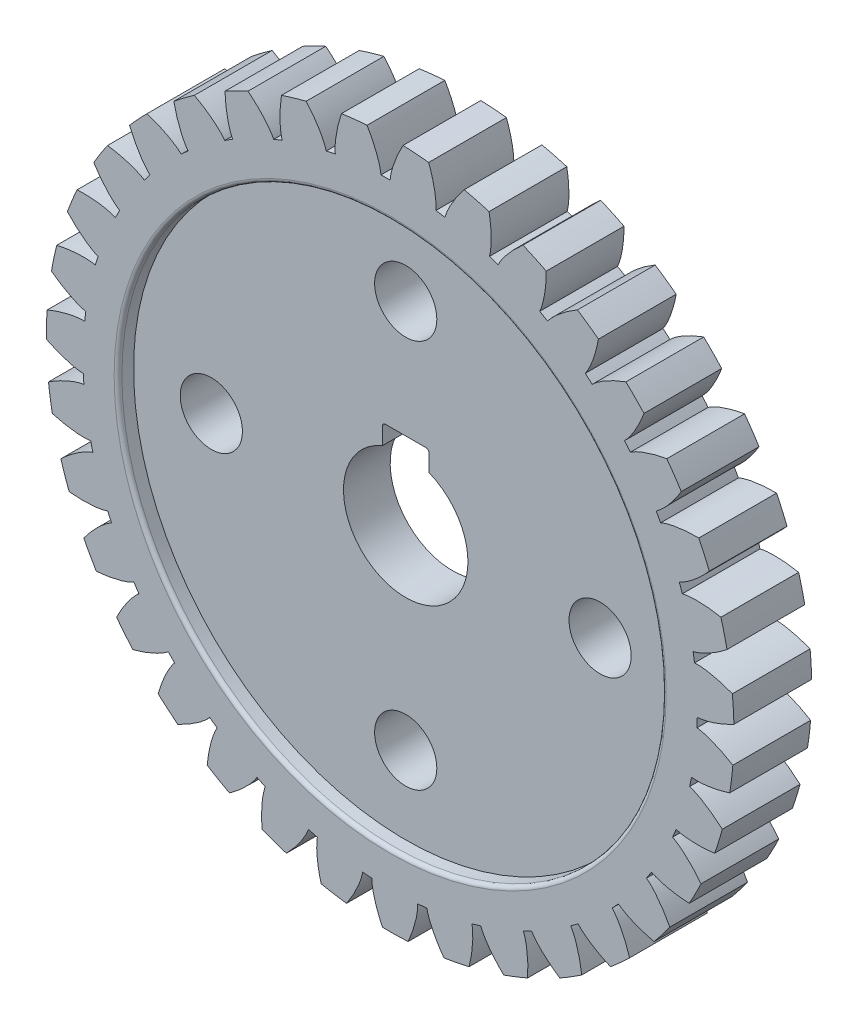
SolidWorks part; units mm, degrees
ref_plane "Front Plane" through (0, 0, 0) normal (0, 0, 1) x (1, 0, 0)
ref_plane "Top Plane" through (0, 0, 0) normal (0, 1, 0) x (1, 0, 0)
ref_plane "Right Plane" through (0, 0, 0) normal (1, 0, 0) x (0, 0, -1)
other "Configuration Table"
sketch "Sketch1" plane through (0, 0, 0) normal (0, 0, 1) x (1, 0, 0)
  line L0 (0, 22.1088) -> (0, 21) construction
  line L1 (0, 0) -> (0.8267, 22.0934) construction
  line L2 (0, 0) -> (2.4754, 21.9698) construction
  line L3 (0, 0) -> (1.6522, 22.047) construction
  line L4 (0, 0) -> (0, 14.7345) construction
  line L5 (0, 0) -> (4.1103, 21.7234) construction
  circle A0 centre (0, 0) radius 22.1088
  circle A1 centre (0, 0) radius 4
  circle A2 centre (0, 0) radius 19.75
  circle A3 centre (0, 0) radius 21 construction
  spline S0 degree 4 poles (0, 19.7335) (0.0004, 19.7495) (0.0024, 19.7944) (0.0107, 19.8789) (0.0304, 20.0163) (0.0799, 20.2697) (0.1609, 20.5699) (0.2731, 20.9038) (0.4141, 21.2564) (0.5474, 21.5537) (0.6917, 21.8458) (0.846, 22.1327) (1.0445, 22.4746) (1.2997, 22.8773) (1.62, 23.3348) (2.0126, 23.8396) (2.4375, 24.3344) (2.883, 24.8087) (3.3503, 25.2649) (3.8321, 25.6999) (4.3364, 26.1194) (4.7811, 26.4645) (5.1863, 26.7575) (5.5052, 26.9802) (5.8044, 27.1773) (6.0923, 27.3663) (6.5858, 27.6653) (6.8965, 27.8456) (7.3865, 28.1155) (7.5689, 28.2075) (7.7138, 28.2832) knots 0 0 0 0 0 0.005377 0.015084 0.028532 0.04661 0.092111 0.119476 0.146842 0.174209 0.201575 0.228941 0.256307 0.307035 0.361767 0.4165 0.471232 0.525964 0.580697 0.635429 0.690161 0.744894 0.77226 0.799626 0.826992 0.854358 0.909091 0.954545 1 1 1 1 1 construction
  spline S1 degree 4 poles (0.0005, 19.75) (0.001, 19.7619) (0.0033, 19.8026) (0.0113, 19.883) (0.0304, 20.0163) (0.0799, 20.2697) (0.1609, 20.5699) (0.2731, 20.9038) (0.4141, 21.2564) (0.5596, 21.5809) (0.6822, 21.8261) (0.7729, 21.9961) (0.8267, 22.0934) knots 0.001383 0.001383 0.001383 0.001383 0.001383 0.005377 0.015084 0.028532 0.04661 0.092111 0.119476 0.146842 0.174209 0.211577 0.211577 0.211577 0.211577 0.211577
  spline S2 degree 4 poles (2.9431, 19.5295) (2.9444, 19.5413) (2.9482, 19.5819) (2.9522, 19.6626) (2.9532, 19.7972) (2.942, 20.0552) (2.9067, 20.3641) (2.8455, 20.711) (2.7586, 21.0808) (2.6631, 21.4232) (2.5785, 21.684) (2.5141, 21.8656) (2.4754, 21.9698) knots 0.001383 0.001383 0.001383 0.001383 0.001383 0.005377 0.015084 0.028532 0.04661 0.092111 0.119476 0.146842 0.174209 0.211577 0.211577 0.211577 0.211577 0.211577
  spline S3 degree 4 poles (4.3953, 19.2547) (4.3984, 19.2662) (4.4097, 19.3054) (4.4354, 19.382) (4.4836, 19.5076) (4.5884, 19.7437) (4.7341, 20.0184) (4.9178, 20.3189) (5.1338, 20.6313) (5.3478, 20.9153) (5.5218, 21.1271) (5.6481, 21.2726) (5.7222, 21.3555) knots 0.001383 0.001383 0.001383 0.001383 0.001383 0.005377 0.015084 0.028532 0.04661 0.092111 0.119476 0.146842 0.174209 0.211577 0.211577 0.211577 0.211577 0.211577
  dimension "D1" = 2.143
  dimension "D2" = 8
  dimension "D3" = 4.286
  dimension "D4" = 42
  dimension "D5" = 6.429
  dimension "D7" = 39.5
  dimension "D6" = 6.429
sketch "Sketch4" plane through (0, 0, 0) normal (0, 0, 1) x (1, 0, 0)
  line L0 (0, 0) -> (4.1103, 21.7234) construction
  line L1 (0, 0) -> (0.7436, 3.9303) construction
  circle A0 centre (0, 0) radius 4 construction
  circle A1 centre (0, 0) radius 4
  arc A2 (0.0005, 19.75) -> (-0.5913, 19.7411) centre (0, 0) ccw
  circle A4 centre (0, 0) radius 19.75 construction
  arc A6 (2.4754, 21.9698) -> (0.8267, 22.0934) centre (0, 0) ccw
  arc A7 (-3.526, 19.4327) -> (-4.1068, 19.3183) centre (0, 0) ccw
  arc A8 (6.3585, 21.1747) -> (4.7583, 21.5907) centre (0, 0) ccw
  arc A9 (10.0372, 19.6991) -> (8.537, 20.3941) centre (0, 0) ccw
  arc A10 (13.3933, 17.5903) -> (12.0413, 18.542) centre (0, 0) ccw
  arc A11 (16.3189, 14.9162) -> (15.1586, 16.094) centre (0, 0) ccw
  arc A12 (18.7201, 11.7626) -> (17.7887, 13.1287) centre (0, 0) ccw
  arc A13 (20.5195, 8.231) -> (19.847, 9.7414) centre (0, 0) ccw
  arc A14 (21.6595, 4.4348) -> (21.2675, 6.041) centre (0, 0) ccw
  arc A15 (22.1032, 0.4961) -> (22.0044, 2.1465) centre (0, 0) ccw
  arc A16 (21.8366, -3.4586) -> (22.034, -1.8171) centre (0, 0) ccw
  arc A17 (20.8681, -7.3021) -> (21.3555, -5.7222) centre (0, 0) ccw
  arc A18 (19.2289, -10.9109) -> (19.9905, -9.4434) centre (0, 0) ccw
  arc A19 (16.9717, -14.169) -> (17.9831, -12.8611) centre (0, 0) ccw
  arc A20 (14.169, -16.9717) -> (15.3977, -15.8654) centre (0, 0) ccw
  arc A21 (10.9109, -19.2289) -> (12.3174, -18.3598) centre (0, 0) ccw
  arc A22 (7.3021, -20.8681) -> (8.8411, -20.2641) centre (0, 0) ccw
  arc A23 (3.4586, -21.8366) -> (5.0808, -21.5171) centre (0, 0) ccw
  arc A24 (-0.4961, -22.1032) -> (1.1571, -22.0785) centre (0, 0) ccw
  arc A25 (-4.4348, -21.6595) -> (-2.8038, -21.9303) centre (0, 0) ccw
  arc A26 (-8.231, -20.5195) -> (-6.6745, -21.0772) centre (0, 0) ccw
  arc A27 (-11.7626, -18.7201) -> (-10.3308, -19.5467) centre (0, 0) ccw
  arc A28 (-14.9162, -16.3189) -> (-13.6549, -17.388) centre (0, 0) ccw
  arc A29 (-17.5903, -13.3933) -> (-16.5402, -14.6704) centre (0, 0) ccw
  arc A30 (-19.6991, -10.0372) -> (-18.8939, -11.4812) centre (0, 0) ccw
  arc A31 (-21.1747, -6.3585) -> (-20.6404, -7.9231) centre (0, 0) ccw
  arc A32 (-21.9698, -2.4754) -> (-21.7234, -4.1103) centre (0, 0) ccw
  arc A33 (-22.0587, 1.4872) -> (-22.1082, -0.1654) centre (0, 0) ccw
  arc A34 (-21.4387, 5.4021) -> (-21.7824, 3.7849) centre (0, 0) ccw
  arc A35 (-20.1296, 9.1433) -> (-20.7566, 7.6134) centre (0, 0) ccw
  arc A36 (-18.1735, 12.5906) -> (-19.0636, 11.1973) centre (0, 0) ccw
  arc A37 (-15.6333, 15.6333) -> (-16.7579, 14.4213) centre (0, 0) ccw
  arc A38 (-12.5906, 18.1735) -> (-13.9135, 17.1818) centre (0, 0) ccw
  arc A39 (-9.1433, 20.1296) -> (-10.622, 19.39) centre (0, 0) ccw
  arc A40 (-5.4021, 21.4387) -> (-6.9891, 20.975) centre (0, 0) ccw
  arc A41 (-1.4872, 22.0587) -> (-3.1315, 21.8859) centre (0, 0) ccw
  arc A42 (3.527, 19.4325) -> (2.9431, 19.5295) centre (0, 0) ccw
  arc A43 (6.9401, 18.4905) -> (6.3829, 18.6901) centre (0, 0) ccw
  arc A44 (10.1302, 16.9541) -> (9.6176, 17.2501) centre (0, 0) ccw
  arc A45 (12.9947, 14.8728) -> (12.5431, 15.2556) centre (0, 0) ccw
  arc A46 (15.4415, 12.3135) -> (15.0656, 12.7707) centre (0, 0) ccw
  arc A47 (17.392, 9.3585) -> (17.1037, 9.8754) centre (0, 0) ccw
  arc A48 (18.7835, 6.1026) -> (18.5922, 6.6628) centre (0, 0) ccw
  arc A49 (19.5713, 2.6506) -> (19.4831, 3.2359) centre (0, 0) ccw
  arc A50 (19.7301, -0.8866) -> (19.7478, -0.2949) centre (0, 0) ccw
  arc A51 (19.2547, -4.3953) -> (19.3778, -3.8163) centre (0, 0) ccw
  arc A52 (18.1605, -7.7627) -> (18.3849, -7.215) centre (0, 0) ccw
  arc A53 (16.4825, -10.8806) -> (16.8012, -10.3818) centre (0, 0) ccw
  arc A54 (14.2748, -13.6489) -> (14.6775, -13.2149) centre (0, 0) ccw
  arc A55 (11.6083, -15.9784) -> (12.082, -15.6233) centre (0, 0) ccw
  arc A56 (8.5687, -17.7944) -> (9.0981, -17.5296) centre (0, 0) ccw
  arc A57 (5.2537, -19.0384) -> (5.8219, -18.8724) centre (0, 0) ccw
  arc A58 (1.7699, -19.6705) -> (2.3585, -19.6087) centre (0, 0) ccw
  arc A59 (-1.7709, -19.6704) -> (-1.1806, -19.7147) centre (0, 0) ccw
  arc A60 (-5.2547, -19.0381) -> (-4.6818, -19.187) centre (0, 0) ccw
  arc A61 (-8.5697, -17.7939) -> (-8.0326, -18.0427) centre (0, 0) ccw
  arc A62 (-11.6092, -15.9778) -> (-11.1251, -16.3185) centre (0, 0) ccw
  arc A63 (-14.2756, -13.6481) -> (-13.8601, -14.0698) centre (0, 0) ccw
  arc A64 (-16.4831, -10.8798) -> (-16.1497, -11.3689) centre (0, 0) ccw
  arc A65 (-18.1609, -7.7618) -> (-17.9201, -8.3025) centre (0, 0) ccw
  arc A66 (-19.2549, -4.3943) -> (-19.1146, -4.9693) centre (0, 0) ccw
  arc A67 (-19.7301, -0.8856) -> (-19.6947, -1.4764) centre (0, 0) ccw
  arc A68 (-19.5712, 2.6516) -> (-19.6419, 2.0639) centre (0, 0) ccw
  arc A69 (-18.7832, 6.1036) -> (-18.9577, 5.5379) centre (0, 0) ccw
  arc A70 (-17.3915, 9.3594) -> (-17.6642, 8.834) centre (0, 0) ccw
  arc A71 (-12.9939, 14.8735) -> (-13.4338, 14.4774) centre (0, 0) ccw
  arc A72 (-15.4409, 12.3143) -> (-15.8029, 11.8461) centre (0, 0) ccw
  arc A73 (-10.1293, 16.9546) -> (-10.6329, 16.6435) centre (0, 0) ccw
  arc A74 (-6.9392, 18.4908) -> (-7.4902, 18.2746) centre (0, 0) ccw
  spline S0 degree 4 poles (3.527, 19.4325) (3.5296, 19.4441) (3.5391, 19.4838) (3.5614, 19.5615) (3.6039, 19.6892) (3.6979, 19.9296) (3.8312, 20.2106) (4.0012, 20.5191) (4.203, 20.8409) (4.404, 21.1342) (4.5684, 21.3536) (4.688, 21.5046) (4.7583, 21.5907) knots 0.001383 0.001383 0.001383 0.001383 0.001383 0.005377 0.015084 0.028532 0.04661 0.092111 0.119476 0.146842 0.174209 0.211577 0.211577 0.211577 0.211577 0.211577
  spline S1 degree 4 poles (-1975.8072, 309.5897) (-30.9922, 20.4545) (1.9661, 17.0455) (2.9426, 18.3846) (2.9532, 19.7972) (2.942, 20.0552) (2.9067, 20.3641) (2.8455, 20.711) (2.7586, 21.0808) (0.373, 29.6398) (-13.398, 34.7339) (17.5347, 27.1799) (-1817.0292, 852.0524) knots -0.428025 -0.428025 -0.428025 -0.428025 -0.428025 0.005377 0.015084 0.028532 0.04661 0.092111 0.119476 0.146842 0.174209 3.077604 3.077604 3.077604 3.077604 3.077604 only from (2.9431, 19.5295) to (2.4754, 21.9698) construction
  spline S2 degree 4 poles (1999.881, 11.6531) (33.6946, 15.6069) (0.5963, 17.1482) (-0.1697, 18.6179) (0.0304, 20.0163) (0.0799, 20.2697) (0.1609, 20.5699) (0.2731, 20.9038) (0.4141, 21.2564) (4.0487, 29.3643) (18.4252, 32.3491) (-13.2879, 29.4898) (1923.7263, 571.7216) knots -0.428025 -0.428025 -0.428025 -0.428025 -0.428025 0.005377 0.015084 0.028532 0.04661 0.092111 0.119476 0.146842 0.174209 3.077604 3.077604 3.077604 3.077604 3.077604 only from (0.0005, 19.75) to (0.8267, 22.0934) construction
  spline S3 degree 4 poles (6.3829, 18.6901) (6.3863, 18.7015) (6.3973, 18.7408) (6.4157, 18.8195) (6.4407, 18.9517) (6.4757, 19.2076) (6.4962, 19.5178) (6.4979, 19.8701) (6.4784, 20.2494) (6.4456, 20.6034) (6.4089, 20.8751) (6.378, 21.0653) (6.3585, 21.1747) knots 0.001383 0.001383 0.001383 0.001383 0.001383 0.005377 0.015084 0.028532 0.04661 0.092111 0.119476 0.146842 0.174209 0.211577 0.211577 0.211577 0.211577 0.211577
  spline S4 degree 4 poles (2.9431, 19.5295) (2.9444, 19.5413) (2.9482, 19.5819) (2.9522, 19.6626) (2.9532, 19.7972) (2.942, 20.0552) (2.9067, 20.3641) (2.8455, 20.711) (2.7586, 21.0808) (2.6631, 21.4232) (2.5785, 21.684) (2.5141, 21.8656) (2.4754, 21.9698) knots 0.001383 0.001383 0.001383 0.001383 0.001383 0.005377 0.015084 0.028532 0.04661 0.092111 0.119476 0.146842 0.174209 0.211577 0.211577 0.211577 0.211577 0.211577
  spline S5 degree 4 poles (0.0005, 19.75) (0.001, 19.7619) (0.0033, 19.8026) (0.0113, 19.883) (0.0304, 20.0163) (0.0799, 20.2697) (0.1609, 20.5699) (0.2731, 20.9038) (0.4141, 21.2564) (0.5596, 21.5809) (0.6822, 21.8261) (0.7729, 21.9961) (0.8267, 22.0934) knots 0.001383 0.001383 0.001383 0.001383 0.001383 0.005377 0.015084 0.028532 0.04661 0.092111 0.119476 0.146842 0.174209 0.211577 0.211577 0.211577 0.211577 0.211577
  spline S6 degree 4 poles (6.9401, 18.4905) (6.9447, 18.5014) (6.9612, 18.5387) (6.997, 18.6112) (7.0616, 18.7292) (7.1971, 18.9491) (7.3783, 19.2017) (7.6007, 19.4749) (7.8567, 19.7555) (8.1069, 20.0082) (8.3078, 20.1947) (8.4524, 20.3219) (8.537, 20.3941) knots 0.001383 0.001383 0.001383 0.001383 0.001383 0.005377 0.015084 0.028532 0.04661 0.092111 0.119476 0.146842 0.174209 0.211577 0.211577 0.211577 0.211577 0.211577
  spline S7 degree 4 poles (9.6176, 17.2501) (9.6229, 17.2607) (9.6408, 17.2973) (9.6729, 17.3715) (9.7212, 17.4971) (9.8013, 17.7426) (9.8768, 18.0442) (9.9414, 18.3905) (9.9899, 18.7672) (10.0209, 19.1214) (10.0333, 19.3953) (10.0368, 19.5879) (10.0372, 19.6991) knots 0.001383 0.001383 0.001383 0.001383 0.001383 0.005377 0.015084 0.028532 0.04661 0.092111 0.119476 0.146842 0.174209 0.211577 0.211577 0.211577 0.211577 0.211577
  spline S8 degree 4 poles (10.1302, 16.9541) (10.1367, 16.9641) (10.1595, 16.9978) (10.2077, 17.0627) (10.2924, 17.1673) (10.4649, 17.3595) (10.6884, 17.5757) (10.956, 17.8048) (11.2579, 18.0352) (11.5492, 18.2391) (11.7802, 18.3867) (11.9452, 18.4861) (12.0413, 18.542) knots 0.001383 0.001383 0.001383 0.001383 0.001383 0.005377 0.015084 0.028532 0.04661 0.092111 0.119476 0.146842 0.174209 0.211577 0.211577 0.211577 0.211577 0.211577
  spline S9 degree 4 poles (12.5431, 15.2556) (12.5503, 15.265) (12.5744, 15.2979) (12.6193, 15.3652) (12.6892, 15.4802) (12.8118, 15.7074) (12.94, 15.9907) (13.0654, 16.3199) (13.1804, 16.6819) (13.2741, 17.0248) (13.3352, 17.2921) (13.3731, 17.481) (13.3933, 17.5903) knots 0.001383 0.001383 0.001383 0.001383 0.001383 0.005377 0.015084 0.028532 0.04661 0.092111 0.119476 0.146842 0.174209 0.211577 0.211577 0.211577 0.211577 0.211577
  spline S10 degree 4 poles (12.9947, 14.8728) (13.0028, 14.8815) (13.0313, 14.9106) (13.0903, 14.9659) (13.1923, 15.0537) (13.3964, 15.2119) (13.6549, 15.3848) (13.9591, 15.5624) (14.2973, 15.7351) (14.6203, 15.8838) (14.874, 15.9878) (15.0541, 16.0561) (15.1586, 16.094) knots 0.001383 0.001383 0.001383 0.001383 0.001383 0.005377 0.015084 0.028532 0.04661 0.092111 0.119476 0.146842 0.174209 0.211577 0.211577 0.211577 0.211577 0.211577
  spline S11 degree 4 poles (15.0656, 12.7707) (15.0743, 12.7788) (15.1039, 12.8068) (15.16, 12.865) (15.2493, 12.9657) (15.4106, 13.1673) (15.5873, 13.4232) (15.7695, 13.7247) (15.9473, 14.0603) (16.1007, 14.3811) (16.2085, 14.6331) (16.2795, 14.8122) (16.3189, 14.9162) knots 0.001383 0.001383 0.001383 0.001383 0.001383 0.005377 0.015084 0.028532 0.04661 0.092111 0.119476 0.146842 0.174209 0.211577 0.211577 0.211577 0.211577 0.211577
  spline S12 degree 4 poles (15.4415, 12.3135) (15.4511, 12.3206) (15.4843, 12.3442) (15.5522, 12.388) (15.6683, 12.4562) (15.8973, 12.5754) (16.1825, 12.6994) (16.5135, 12.8198) (16.8772, 12.9294) (17.2215, 13.018) (17.4897, 13.075) (17.6791, 13.1101) (17.7887, 13.1287) knots 0.001383 0.001383 0.001383 0.001383 0.001383 0.005377 0.015084 0.028532 0.04661 0.092111 0.119476 0.146842 0.174209 0.211577 0.211577 0.211577 0.211577 0.211577
  spline S13 degree 4 poles (17.1037, 9.8754) (17.1138, 9.8818) (17.1479, 9.9041) (17.2135, 9.9513) (17.3194, 10.0344) (17.5141, 10.2041) (17.7336, 10.4242) (17.9667, 10.6884) (18.2015, 10.9869) (18.4098, 11.2751) (18.5609, 11.5038) (18.6627, 11.6673) (18.7201, 11.7626) knots 0.001383 0.001383 0.001383 0.001383 0.001383 0.005377 0.015084 0.028532 0.04661 0.092111 0.119476 0.146842 0.174209 0.211577 0.211577 0.211577 0.211577 0.211577
  spline S14 degree 4 poles (17.392, 9.3585) (17.4027, 9.3637) (17.4396, 9.3809) (17.5142, 9.412) (17.6406, 9.4583) (17.8873, 9.5348) (18.19, 9.6058) (18.5372, 9.6652) (18.9146, 9.7081) (19.2692, 9.7337) (19.5432, 9.742) (19.7359, 9.7427) (19.847, 9.7414) knots 0.001383 0.001383 0.001383 0.001383 0.001383 0.005377 0.015084 0.028532 0.04661 0.092111 0.119476 0.146842 0.174209 0.211577 0.211577 0.211577 0.211577 0.211577
  spline S15 degree 4 poles (18.5922, 6.6628) (18.6032, 6.6672) (18.6408, 6.6831) (18.7138, 6.7178) (18.8328, 6.7807) (19.0546, 6.9128) (19.31, 7.0903) (19.5864, 7.3086) (19.8708, 7.5603) (20.1272, 7.8067) (20.3167, 8.0048) (20.4461, 8.1475) (20.5195, 8.231) knots 0.001383 0.001383 0.001383 0.001383 0.001383 0.005377 0.015084 0.028532 0.04661 0.092111 0.119476 0.146842 0.174209 0.211577 0.211577 0.211577 0.211577 0.211577
  spline S16 degree 4 poles (18.7835, 6.1026) (18.795, 6.1058) (18.8344, 6.1162) (18.9134, 6.1334) (19.046, 6.1565) (19.3023, 6.1877) (19.6128, 6.2035) (19.9651, 6.1999) (20.3441, 6.1747) (20.6976, 6.1367) (20.9687, 6.0959) (21.1583, 6.0621) (21.2675, 6.041) knots 0.001383 0.001383 0.001383 0.001383 0.001383 0.005377 0.015084 0.028532 0.04661 0.092111 0.119476 0.146842 0.174209 0.211577 0.211577 0.211577 0.211577 0.211577
  spline S17 degree 4 poles (19.4831, 3.2359) (19.4947, 3.2383) (19.5345, 3.2472) (19.6125, 3.2684) (19.7409, 3.309) (19.9827, 3.3994) (20.2657, 3.5284) (20.5767, 3.6938) (20.9014, 3.8907) (21.1977, 4.0874) (21.4195, 4.2485) (21.5723, 4.3658) (21.6595, 4.4348) knots 0.001383 0.001383 0.001383 0.001383 0.001383 0.005377 0.015084 0.028532 0.04661 0.092111 0.119476 0.146842 0.174209 0.211577 0.211577 0.211577 0.211577 0.211577
  spline S18 degree 4 poles (19.5713, 2.6506) (19.5832, 2.6517) (19.6238, 2.6549) (19.7046, 2.6578) (19.8392, 2.6567) (20.0969, 2.6417) (20.4053, 2.6018) (20.7513, 2.5354) (21.1197, 2.4429) (21.4607, 2.3423) (21.7202, 2.2538) (21.9007, 2.1867) (22.0044, 2.1465) knots 0.001383 0.001383 0.001383 0.001383 0.001383 0.005377 0.015084 0.028532 0.04661 0.092111 0.119476 0.146842 0.174209 0.211577 0.211577 0.211577 0.211577 0.211577
  spline S19 degree 4 poles (19.7478, -0.2949) (19.7597, -0.2946) (19.8004, -0.293) (19.8809, -0.2861) (20.0145, -0.2691) (20.2686, -0.2233) (20.57, -0.1469) (20.9055, -0.0396) (21.2603, 0.0961) (21.5868, 0.2367) (21.8339, 0.3556) (22.0052, 0.4437) (22.1032, 0.4961) knots 0.001383 0.001383 0.001383 0.001383 0.001383 0.005377 0.015084 0.028532 0.04661 0.092111 0.119476 0.146842 0.174209 0.211577 0.211577 0.211577 0.211577 0.211577
  spline S20 degree 4 poles (19.7301, -0.8866) (19.7419, -0.8876) (19.7825, -0.8917) (19.8625, -0.9033) (19.9947, -0.9284) (20.2457, -0.9892) (20.542, -1.0836) (20.8705, -1.2107) (21.2165, -1.3674) (21.534, -1.5272) (21.7735, -1.6607) (21.9392, -1.7589) (22.034, -1.8171) knots 0.001383 0.001383 0.001383 0.001383 0.001383 0.005377 0.015084 0.028532 0.04661 0.092111 0.119476 0.146842 0.174209 0.211577 0.211577 0.211577 0.211577 0.211577
  spline S21 degree 4 poles (19.3778, -3.8163) (19.3895, -3.8181) (19.4299, -3.8238) (19.5104, -3.8314) (19.6448, -3.8385) (19.903, -3.8388) (20.2132, -3.8174) (20.5625, -3.7718) (20.9358, -3.7016) (21.2822, -3.6216) (21.5465, -3.5487) (21.7307, -3.4926) (21.8366, -3.4586) knots 0.001383 0.001383 0.001383 0.001383 0.001383 0.005377 0.015084 0.028532 0.04661 0.092111 0.119476 0.146842 0.174209 0.211577 0.211577 0.211577 0.211577 0.211577
  spline S22 degree 4 poles (19.2547, -4.3953) (19.2662, -4.3984) (19.3054, -4.4097) (19.382, -4.4354) (19.5076, -4.4836) (19.7437, -4.5884) (20.0184, -4.7341) (20.3189, -4.9178) (20.6313, -5.1338) (20.9153, -5.3478) (21.1271, -5.5218) (21.2726, -5.6481) (21.3555, -5.7222) knots 0.001383 0.001383 0.001383 0.001383 0.001383 0.005377 0.015084 0.028532 0.04661 0.092111 0.119476 0.146842 0.174209 0.211577 0.211577 0.211577 0.211577 0.211577
  spline S23 degree 4 poles (18.3849, -7.215) (18.3962, -7.2189) (18.4349, -7.2317) (18.5127, -7.2535) (18.6437, -7.2845) (18.8977, -7.3309) (19.2067, -7.3653) (19.5586, -7.3828) (19.9384, -7.3803) (20.2935, -7.3635) (20.5666, -7.339) (20.7579, -7.3166) (20.8681, -7.3021) knots 0.001383 0.001383 0.001383 0.001383 0.001383 0.005377 0.015084 0.028532 0.04661 0.092111 0.119476 0.146842 0.174209 0.211577 0.211577 0.211577 0.211577 0.211577
  spline S24 degree 4 poles (18.1605, -7.7627) (18.1712, -7.7678) (18.2077, -7.7859) (18.2785, -7.8249) (18.3936, -7.8948) (18.6071, -8.04) (18.8514, -8.2324) (19.1143, -8.4668) (19.3831, -8.7351) (19.6243, -8.9964) (19.8016, -9.2055) (19.9222, -9.3557) (19.9905, -9.4434) knots 0.001383 0.001383 0.001383 0.001383 0.001383 0.005377 0.015084 0.028532 0.04661 0.092111 0.119476 0.146842 0.174209 0.211577 0.211577 0.211577 0.211577 0.211577
  spline S25 degree 4 poles (16.8012, -10.3818) (16.8116, -10.3877) (16.8474, -10.4071) (16.92, -10.4425) (17.0434, -10.4964) (17.285, -10.5874) (17.583, -10.6764) (17.926, -10.7565) (18.3001, -10.8219) (18.6526, -10.8687) (18.9256, -10.8933) (19.1179, -10.9055) (19.2289, -10.9109) knots 0.001383 0.001383 0.001383 0.001383 0.001383 0.005377 0.015084 0.028532 0.04661 0.092111 0.119476 0.146842 0.174209 0.211577 0.211577 0.211577 0.211577 0.211577
  spline S26 degree 4 poles (16.4825, -10.8806) (16.4922, -10.8876) (16.5249, -10.9119) (16.5876, -10.9629) (16.6883, -11.0522) (16.8725, -11.2332) (17.0785, -11.4661) (17.2953, -11.7438) (17.5119, -12.0557) (17.7026, -12.3559) (17.8397, -12.5933) (17.9315, -12.7626) (17.9831, -12.8611) knots 0.001383 0.001383 0.001383 0.001383 0.001383 0.005377 0.015084 0.028532 0.04661 0.092111 0.119476 0.146842 0.174209 0.211577 0.211577 0.211577 0.211577 0.211577
  spline S27 degree 4 poles (14.6775, -13.2149) (14.6866, -13.2225) (14.7184, -13.2481) (14.7835, -13.2959) (14.8953, -13.3709) (15.1168, -13.5037) (15.394, -13.6444) (15.7173, -13.7844) (16.0737, -13.9156) (16.4122, -14.0246) (16.6764, -14.0976) (16.8634, -14.1439) (16.9717, -14.169) knots 0.001383 0.001383 0.001383 0.001383 0.001383 0.005377 0.015084 0.028532 0.04661 0.092111 0.119476 0.146842 0.174209 0.211577 0.211577 0.211577 0.211577 0.211577
  spline S28 degree 4 poles (14.2748, -13.6489) (14.2831, -13.6574) (14.3109, -13.6872) (14.3635, -13.7486) (14.4467, -13.8544) (14.5956, -14.0654) (14.7567, -14.3313) (14.9204, -14.6432) (15.0778, -14.9889) (15.2118, -15.3182) (15.3044, -15.5763) (15.3645, -15.7593) (15.3977, -15.8654) knots 0.001383 0.001383 0.001383 0.001383 0.001383 0.005377 0.015084 0.028532 0.04661 0.092111 0.119476 0.146842 0.174209 0.211577 0.211577 0.211577 0.211577 0.211577
  spline S29 degree 4 poles (12.082, -15.6233) (12.0896, -15.6324) (12.1163, -15.6632) (12.1719, -15.7219) (12.2685, -15.8157) (12.4627, -15.9858) (12.7104, -16.1738) (13.0034, -16.3693) (13.3307, -16.562) (13.6442, -16.7297) (13.8912, -16.8487) (14.0669, -16.9277) (14.169, -16.9717) knots 0.001383 0.001383 0.001383 0.001383 0.001383 0.005377 0.015084 0.028532 0.04661 0.092111 0.119476 0.146842 0.174209 0.211577 0.211577 0.211577 0.211577 0.211577
  spline S30 degree 4 poles (11.6083, -15.9784) (11.6149, -15.9883) (11.637, -16.0225) (11.6778, -16.0923) (11.7407, -16.2113) (11.8495, -16.4455) (11.9605, -16.7359) (12.066, -17.072) (12.1592, -17.4403) (12.2322, -17.7882) (12.2772, -18.0587) (12.3037, -18.2495) (12.3174, -18.3598) knots 0.001383 0.001383 0.001383 0.001383 0.001383 0.005377 0.015084 0.028532 0.04661 0.092111 0.119476 0.146842 0.174209 0.211577 0.211577 0.211577 0.211577 0.211577
  spline S31 degree 4 poles (9.0981, -17.5296) (9.104, -17.5399) (9.1248, -17.575) (9.169, -17.6427) (9.2473, -17.7521) (9.408, -17.9542) (9.6181, -18.1834) (9.8716, -18.4281) (10.1592, -18.6761) (10.4378, -18.8971) (10.6595, -19.0583) (10.8183, -19.1674) (10.9109, -19.2289) knots 0.001383 0.001383 0.001383 0.001383 0.001383 0.005377 0.015084 0.028532 0.04661 0.092111 0.119476 0.146842 0.174209 0.211577 0.211577 0.211577 0.211577 0.211577
  spline S32 degree 4 poles (8.5687, -17.7944) (8.5735, -17.8053) (8.5891, -17.8429) (8.6167, -17.9189) (8.6574, -18.0472) (8.7227, -18.297) (8.78, -18.6026) (8.8238, -18.9522) (8.8497, -19.3311) (8.8594, -19.6865) (8.8554, -19.9606) (8.8474, -20.1531) (8.8411, -20.2641) knots 0.001383 0.001383 0.001383 0.001383 0.001383 0.005377 0.015084 0.028532 0.04661 0.092111 0.119476 0.146842 0.174209 0.211577 0.211577 0.211577 0.211577 0.211577
  spline S33 degree 4 poles (5.8219, -18.8724) (5.8259, -18.8836) (5.84, -18.9218) (5.8714, -18.9963) (5.9289, -19.118) (6.051, -19.3456) (6.2168, -19.6086) (6.4225, -19.8946) (6.6612, -20.19) (6.8958, -20.4572) (7.0852, -20.6554) (7.222, -20.791) (7.3021, -20.8681) knots 0.001383 0.001383 0.001383 0.001383 0.001383 0.005377 0.015084 0.028532 0.04661 0.092111 0.119476 0.146842 0.174209 0.211577 0.211577 0.211577 0.211577 0.211577
  spline S34 degree 4 poles (5.2537, -19.0384) (5.2564, -19.05) (5.2651, -19.0898) (5.2787, -19.1695) (5.2958, -19.303) (5.3154, -19.5605) (5.3173, -19.8714) (5.2979, -20.2231) (5.2558, -20.6006) (5.2019, -20.952) (5.149, -21.221) (5.1068, -21.409) (5.0808, -21.5171) knots 0.001383 0.001383 0.001383 0.001383 0.001383 0.005377 0.015084 0.028532 0.04661 0.092111 0.119476 0.146842 0.174209 0.211577 0.211577 0.211577 0.211577 0.211577
  spline S35 degree 4 poles (2.3585, -19.6087) (2.3604, -19.6204) (2.3675, -19.6605) (2.3851, -19.7394) (2.42, -19.8694) (2.4994, -20.1151) (2.6156, -20.4035) (2.7669, -20.7217) (2.9491, -21.0549) (3.1322, -21.3597) (3.2832, -21.5885) (3.3935, -21.7464) (3.4586, -21.8366) knots 0.001383 0.001383 0.001383 0.001383 0.001383 0.005377 0.015084 0.028532 0.04661 0.092111 0.119476 0.146842 0.174209 0.211577 0.211577 0.211577 0.211577 0.211577
  spline S36 degree 4 poles (1.7699, -19.6705) (1.7705, -19.6824) (1.7718, -19.7231) (1.771, -19.804) (1.764, -19.9384) (1.7373, -20.1952) (1.6837, -20.5015) (1.6018, -20.8441) (1.4929, -21.208) (1.3772, -21.5442) (1.2771, -21.7994) (1.202, -21.9768) (1.1571, -22.0785) knots 0.001383 0.001383 0.001383 0.001383 0.001383 0.005377 0.015084 0.028532 0.04661 0.092111 0.119476 0.146842 0.174209 0.211577 0.211577 0.211577 0.211577 0.211577
  spline S37 degree 4 poles (-1.1806, -19.7147) (-1.1809, -19.7266) (-1.181, -19.7673) (-1.1778, -19.8481) (-1.1667, -19.9822) (-1.1324, -20.2382) (-1.0696, -20.5427) (-0.9775, -20.8827) (-0.8578, -21.2432) (-0.732, -21.5757) (-0.6244, -21.8278) (-0.544, -22.0029) (-0.4961, -22.1032) knots 0.001383 0.001383 0.001383 0.001383 0.001383 0.005377 0.015084 0.028532 0.04661 0.092111 0.119476 0.146842 0.174209 0.211577 0.211577 0.211577 0.211577 0.211577
  spline S38 degree 4 poles (-1.7709, -19.6704) (-1.7724, -19.6822) (-1.7783, -19.7226) (-1.7936, -19.8019) (-1.8245, -19.9329) (-1.8966, -20.1809) (-2.0041, -20.4727) (-2.1458, -20.7952) (-2.3179, -21.1337) (-2.4918, -21.4438) (-2.6359, -21.6771) (-2.7415, -21.8382) (-2.8038, -21.9303) knots 0.001383 0.001383 0.001383 0.001383 0.001383 0.005377 0.015084 0.028532 0.04661 0.092111 0.119476 0.146842 0.174209 0.211577 0.211577 0.211577 0.211577 0.211577
  spline S39 degree 4 poles (-4.6818, -19.187) (-4.6842, -19.1987) (-4.6916, -19.2388) (-4.7029, -19.3188) (-4.716, -19.4528) (-4.7279, -19.7107) (-4.7205, -20.0216) (-4.6906, -20.3726) (-4.6371, -20.7486) (-4.5728, -21.0983) (-4.5118, -21.3656) (-4.464, -21.5522) (-4.4348, -21.6595) knots 0.001383 0.001383 0.001383 0.001383 0.001383 0.005377 0.015084 0.028532 0.04661 0.092111 0.119476 0.146842 0.174209 0.211577 0.211577 0.211577 0.211577 0.211577
  spline S40 degree 4 poles (-5.2547, -19.0381) (-5.2583, -19.0494) (-5.2714, -19.0881) (-5.3005, -19.1635) (-5.3543, -19.2868) (-5.4695, -19.5179) (-5.6274, -19.7858) (-5.8244, -20.0778) (-6.0542, -20.3802) (-6.2807, -20.6543) (-6.4641, -20.8581) (-6.5968, -20.9978) (-6.6745, -21.0772) knots 0.001383 0.001383 0.001383 0.001383 0.001383 0.005377 0.015084 0.028532 0.04661 0.092111 0.119476 0.146842 0.174209 0.211577 0.211577 0.211577 0.211577 0.211577
  spline S41 degree 4 poles (-8.0326, -18.0427) (-8.037, -18.0538) (-8.0515, -18.0919) (-8.0768, -18.1686) (-8.1136, -18.2981) (-8.1714, -18.5498) (-8.2196, -18.857) (-8.2529, -19.2076) (-8.2674, -19.5872) (-8.2665, -19.9427) (-8.2543, -20.2166) (-8.2406, -20.4087) (-8.231, -20.5195) knots 0.001383 0.001383 0.001383 0.001383 0.001383 0.005377 0.015084 0.028532 0.04661 0.092111 0.119476 0.146842 0.174209 0.211577 0.211577 0.211577 0.211577 0.211577
  spline S42 degree 4 poles (-8.5697, -17.7939) (-8.5752, -17.8044) (-8.595, -17.8401) (-8.6371, -17.9091) (-8.7121, -18.0208) (-8.8667, -18.2277) (-9.0699, -18.463) (-9.3159, -18.7152) (-9.596, -18.9717) (-9.8678, -19.2009) (-10.0846, -19.3687) (-10.2401, -19.4824) (-10.3308, -19.5467) knots 0.001383 0.001383 0.001383 0.001383 0.001383 0.005377 0.015084 0.028532 0.04661 0.092111 0.119476 0.146842 0.174209 0.211577 0.211577 0.211577 0.211577 0.211577
  spline S43 degree 4 poles (-11.1251, -16.3185) (-11.1314, -16.3286) (-11.1525, -16.3635) (-11.1911, -16.4345) (-11.2505, -16.5553) (-11.3523, -16.7926) (-11.4545, -17.0863) (-11.5499, -17.4254) (-11.632, -17.7962) (-11.6946, -18.1462) (-11.7315, -18.4179) (-11.7522, -18.6094) (-11.7626, -18.7201) knots 0.001383 0.001383 0.001383 0.001383 0.001383 0.005377 0.015084 0.028532 0.04661 0.092111 0.119476 0.146842 0.174209 0.211577 0.211577 0.211577 0.211577 0.211577
  spline S44 degree 4 poles (-11.6092, -15.9778) (-11.6165, -15.9871) (-11.6423, -16.0187) (-11.6961, -16.079) (-11.7898, -16.1756) (-11.9789, -16.3515) (-12.2208, -16.5468) (-12.5079, -16.751) (-12.8293, -16.9534) (-13.1376, -17.1304) (-13.3809, -17.2567) (-13.5542, -17.3409) (-13.6549, -17.388) knots 0.001383 0.001383 0.001383 0.001383 0.001383 0.005377 0.015084 0.028532 0.04661 0.092111 0.119476 0.146842 0.174209 0.211577 0.211577 0.211577 0.211577 0.211577
  spline S45 degree 4 poles (-13.8601, -14.0698) (-13.8681, -14.0786) (-13.8951, -14.1092) (-13.9458, -14.1721) (-14.0257, -14.2804) (-14.1683, -14.4957) (-14.3213, -14.7664) (-14.4757, -15.083) (-14.6227, -15.4332) (-14.7468, -15.7664) (-14.8316, -16.0271) (-14.8862, -16.2119) (-14.9162, -16.3189) knots 0.001383 0.001383 0.001383 0.001383 0.001383 0.005377 0.015084 0.028532 0.04661 0.092111 0.119476 0.146842 0.174209 0.211577 0.211577 0.211577 0.211577 0.211577
  spline S46 degree 4 poles (-14.2756, -13.6481) (-14.2845, -13.656) (-14.3154, -13.6825) (-14.3791, -13.7322) (-14.4886, -13.8105) (-14.706, -13.9498) (-14.979, -14.0988) (-15.2979, -14.2484) (-15.6503, -14.3902) (-15.9853, -14.5093) (-16.2472, -14.5902) (-16.4327, -14.642) (-16.5402, -14.6704) knots 0.001383 0.001383 0.001383 0.001383 0.001383 0.005377 0.015084 0.028532 0.04661 0.092111 0.119476 0.146842 0.174209 0.211577 0.211577 0.211577 0.211577 0.211577
  spline S47 degree 4 poles (-16.1497, -11.3689) (-16.1591, -11.3761) (-16.1911, -11.4014) (-16.2522, -11.4542) (-16.3502, -11.5465) (-16.5289, -11.7329) (-16.7278, -11.9719) (-16.9362, -12.2559) (-17.1434, -12.5742) (-17.325, -12.8799) (-17.455, -13.1213) (-17.5417, -13.2933) (-17.5903, -13.3933) knots 0.001383 0.001383 0.001383 0.001383 0.001383 0.005377 0.015084 0.028532 0.04661 0.092111 0.119476 0.146842 0.174209 0.211577 0.211577 0.211577 0.211577 0.211577
  spline S48 degree 4 poles (-16.4831, -10.8798) (-16.4933, -10.8859) (-16.5285, -10.9065) (-16.6001, -10.944) (-16.7218, -11.0015) (-16.9606, -11.0998) (-17.2557, -11.1976) (-17.5962, -11.2879) (-17.9682, -11.3645) (-18.3191, -11.4218) (-18.5913, -11.4546) (-18.7831, -11.4725) (-18.8939, -11.4812) knots 0.001383 0.001383 0.001383 0.001383 0.001383 0.005377 0.015084 0.028532 0.04661 0.092111 0.119476 0.146842 0.174209 0.211577 0.211577 0.211577 0.211577 0.211577
  spline S49 degree 4 poles (-17.9201, -8.3025) (-17.9307, -8.3079) (-17.9667, -8.3271) (-18.0363, -8.3682) (-18.1492, -8.4415) (-18.3583, -8.593) (-18.5967, -8.7927) (-18.8525, -9.0349) (-19.1131, -9.3111) (-19.3464, -9.5794) (-19.5174, -9.7937) (-19.6334, -9.9475) (-19.6991, -10.0372) knots 0.001383 0.001383 0.001383 0.001383 0.001383 0.005377 0.015084 0.028532 0.04661 0.092111 0.119476 0.146842 0.174209 0.211577 0.211577 0.211577 0.211577 0.211577
  spline S50 degree 4 poles (-18.1609, -7.7618) (-18.172, -7.766) (-18.2103, -7.7799) (-18.2874, -7.8041) (-18.4174, -7.839) (-18.6699, -7.893) (-18.9778, -7.9366) (-19.329, -7.9646) (-19.7087, -7.9735) (-20.0642, -7.9673) (-20.3378, -7.9509) (-20.5297, -7.9343) (-20.6404, -7.9231) knots 0.001383 0.001383 0.001383 0.001383 0.001383 0.005377 0.015084 0.028532 0.04661 0.092111 0.119476 0.146842 0.174209 0.211577 0.211577 0.211577 0.211577 0.211577
  spline S51 degree 4 poles (-19.1146, -4.9693) (-19.126, -4.9728) (-19.1648, -4.9852) (-19.2406, -5.0132) (-19.3648, -5.0652) (-19.5976, -5.1769) (-19.8678, -5.3308) (-20.1627, -5.5234) (-20.4685, -5.7487) (-20.7459, -5.9711) (-20.9524, -6.1514) (-21.0941, -6.2819) (-21.1747, -6.3585) knots 0.001383 0.001383 0.001383 0.001383 0.001383 0.005377 0.015084 0.028532 0.04661 0.092111 0.119476 0.146842 0.174209 0.211577 0.211577 0.211577 0.211577 0.211577
  spline S52 degree 4 poles (-19.2549, -4.3943) (-19.2666, -4.3965) (-19.3068, -4.4033) (-19.387, -4.4134) (-19.5212, -4.4244) (-19.7792, -4.4325) (-20.09, -4.4204) (-20.4405, -4.3853) (-20.8157, -4.3262) (-21.1643, -4.2566) (-21.4307, -4.1917) (-21.6165, -4.1411) (-21.7234, -4.1103) knots 0.001383 0.001383 0.001383 0.001383 0.001383 0.005377 0.015084 0.028532 0.04661 0.092111 0.119476 0.146842 0.174209 0.211577 0.211577 0.211577 0.211577 0.211577
  spline S53 degree 4 poles (-19.6947, -1.4764) (-19.7065, -1.4778) (-19.747, -1.4831) (-19.8266, -1.4971) (-19.958, -1.5261) (-20.207, -1.5945) (-20.5004, -1.6976) (-20.8249, -1.8345) (-21.1661, -2.0015) (-21.4787, -2.1708) (-21.7141, -2.3113) (-21.8768, -2.4145) (-21.9698, -2.4754) knots 0.001383 0.001383 0.001383 0.001383 0.001383 0.005377 0.015084 0.028532 0.04661 0.092111 0.119476 0.146842 0.174209 0.211577 0.211577 0.211577 0.211577 0.211577
  spline S54 degree 4 poles (-19.7301, -0.8856) (-19.742, -0.8856) (-19.7828, -0.8852) (-19.8635, -0.8807) (-19.9975, -0.8677) (-20.2528, -0.8295) (-20.5564, -0.7622) (-20.895, -0.665) (-21.2536, -0.5399) (-21.5843, -0.4092) (-21.8347, -0.2978) (-22.0086, -0.2148) (-22.1082, -0.1654) knots 0.001383 0.001383 0.001383 0.001383 0.001383 0.005377 0.015084 0.028532 0.04661 0.092111 0.119476 0.146842 0.174209 0.211577 0.211577 0.211577 0.211577 0.211577
  spline S55 degree 4 poles (-19.6419, 2.0639) (-19.6537, 2.0647) (-19.6944, 2.0667) (-19.7753, 2.0671) (-19.9098, 2.0621) (-20.167, 2.0393) (-20.474, 1.9902) (-20.8178, 1.9134) (-21.1833, 1.81) (-21.5212, 1.6993) (-21.7779, 1.603) (-21.9563, 1.5306) (-22.0587, 1.4872) knots 0.001383 0.001383 0.001383 0.001383 0.001383 0.005377 0.015084 0.028532 0.04661 0.092111 0.119476 0.146842 0.174209 0.211577 0.211577 0.211577 0.211577 0.211577
  spline S56 degree 4 poles (-19.5712, 2.6516) (-19.5829, 2.6537) (-19.6229, 2.6614) (-19.7015, 2.6802) (-19.831, 2.7169) (-20.0755, 2.8001) (-20.3621, 2.9206) (-20.678, 3.0766) (-21.0085, 3.2637) (-21.3105, 3.4514) (-21.537, 3.6058) (-21.6932, 3.7185) (-21.7824, 3.7849) knots 0.001383 0.001383 0.001383 0.001383 0.001383 0.005377 0.015084 0.028532 0.04661 0.092111 0.119476 0.146842 0.174209 0.211577 0.211577 0.211577 0.211577 0.211577
  spline S57 degree 4 poles (-18.9577, 5.5379) (-18.9692, 5.5408) (-19.0089, 5.5501) (-19.0884, 5.5649) (-19.2216, 5.5839) (-19.4788, 5.6074) (-19.7896, 5.614) (-20.1416, 5.5999) (-20.5197, 5.5634) (-20.8719, 5.5147) (-21.1416, 5.4659) (-21.3302, 5.4264) (-21.4387, 5.4021) knots 0.001383 0.001383 0.001383 0.001383 0.001383 0.005377 0.015084 0.028532 0.04661 0.092111 0.119476 0.146842 0.174209 0.211577 0.211577 0.211577 0.211577 0.211577
  spline S58 degree 4 poles (-18.7832, 6.1036) (-18.7944, 6.1077) (-18.8324, 6.1224) (-18.9064, 6.1549) (-19.0272, 6.2142) (-19.2529, 6.3397) (-19.5134, 6.5094) (-19.7963, 6.7194) (-20.0881, 6.9625) (-20.3517, 7.2011) (-20.5471, 7.3934) (-20.6807, 7.5322) (-20.7566, 7.6134) knots 0.001383 0.001383 0.001383 0.001383 0.001383 0.005377 0.015084 0.028532 0.04661 0.092111 0.119476 0.146842 0.174209 0.211577 0.211577 0.211577 0.211577 0.211577
  spline S59 degree 4 poles (-17.6642, 8.834) (-17.675, 8.8389) (-17.7124, 8.855) (-17.788, 8.8838) (-17.9157, 8.9264) (-18.1645, 8.9954) (-18.4692, 9.0573) (-18.818, 9.1063) (-19.1965, 9.1379) (-19.5518, 9.1529) (-19.8259, 9.153) (-20.0185, 9.1479) (-20.1296, 9.1433) knots 0.001383 0.001383 0.001383 0.001383 0.001383 0.005377 0.015084 0.028532 0.04661 0.092111 0.119476 0.146842 0.174209 0.211577 0.211577 0.211577 0.211577 0.211577
  spline S60 degree 4 poles (-17.3915, 9.3594) (-17.4017, 9.3654) (-17.4365, 9.3867) (-17.5035, 9.4319) (-17.6118, 9.5118) (-17.8115, 9.6755) (-18.0375, 9.8891) (-18.2784, 10.1461) (-18.5221, 10.4375) (-18.7389, 10.7193) (-18.8967, 10.9434) (-19.0034, 11.1038) (-19.0636, 11.1973) knots 0.001383 0.001383 0.001383 0.001383 0.001383 0.005377 0.015084 0.028532 0.04661 0.092111 0.119476 0.146842 0.174209 0.211577 0.211577 0.211577 0.211577 0.211577
  spline S61 degree 4 poles (-15.8029, 11.8461) (-15.8127, 11.8528) (-15.8467, 11.8754) (-15.9158, 11.9172) (-16.0339, 11.9819) (-16.2664, 12.0942) (-16.5551, 12.2096) (-16.8896, 12.32) (-17.2564, 12.4187) (-17.6032, 12.4969) (-17.873, 12.546) (-18.0634, 12.5753) (-18.1735, 12.5906) knots 0.001383 0.001383 0.001383 0.001383 0.001383 0.005377 0.015084 0.028532 0.04661 0.092111 0.119476 0.146842 0.174209 0.211577 0.211577 0.211577 0.211577 0.211577
  spline S62 degree 4 poles (-15.4409, 12.3143) (-15.4498, 12.3221) (-15.4802, 12.3492) (-15.5381, 12.4057) (-15.6304, 12.5037) (-15.7976, 12.7004) (-15.9819, 12.9509) (-16.173, 13.2468) (-16.3607, 13.577) (-16.5237, 13.893) (-16.639, 14.1417) (-16.7153, 14.3186) (-16.7579, 14.4213) knots 0.001383 0.001383 0.001383 0.001383 0.001383 0.005377 0.015084 0.028532 0.04661 0.092111 0.119476 0.146842 0.174209 0.211577 0.211577 0.211577 0.211577 0.211577
  spline S63 degree 4 poles (-13.4338, 14.4774) (-13.4422, 14.4858) (-13.4716, 14.5141) (-13.5322, 14.5676) (-13.6368, 14.6523) (-13.8455, 14.8043) (-14.109, 14.9694) (-14.4184, 15.1378) (-14.7616, 15.3004) (-15.0889, 15.4393) (-15.3456, 15.5357) (-15.5277, 15.5986) (-15.6333, 15.6333) knots 0.001383 0.001383 0.001383 0.001383 0.001383 0.005377 0.015084 0.028532 0.04661 0.092111 0.119476 0.146842 0.174209 0.211577 0.211577 0.211577 0.211577 0.211577
  spline S64 degree 4 poles (-12.9939, 14.8735) (-13.0014, 14.8828) (-13.0264, 14.9149) (-13.0733, 14.9808) (-13.1466, 15.0937) (-13.276, 15.3171) (-13.4126, 15.5964) (-13.5478, 15.9217) (-13.6736, 16.2801) (-13.7775, 16.6201) (-13.8465, 16.8854) (-13.89, 17.0731) (-13.9135, 17.1818) knots 0.001383 0.001383 0.001383 0.001383 0.001383 0.005377 0.015084 0.028532 0.04661 0.092111 0.119476 0.146842 0.174209 0.211577 0.211577 0.211577 0.211577 0.211577
  spline S65 degree 4 poles (-10.6329, 16.6435) (-10.6396, 16.6532) (-10.6635, 16.6863) (-10.7136, 16.7497) (-10.8014, 16.8518) (-10.9795, 17.0386) (-11.2094, 17.2481) (-11.4837, 17.4691) (-11.7924, 17.6903) (-12.0897, 17.8854) (-12.325, 18.0261) (-12.4929, 18.1205) (-12.5906, 18.1735) knots 0.001383 0.001383 0.001383 0.001383 0.001383 0.005377 0.015084 0.028532 0.04661 0.092111 0.119476 0.146842 0.174209 0.211577 0.211577 0.211577 0.211577 0.211577
  spline S66 degree 4 poles (-10.1293, 16.9546) (-10.135, 16.9651) (-10.1539, 17.0012) (-10.1883, 17.0743) (-10.2402, 17.1985) (-10.3277, 17.4415) (-10.4122, 17.7407) (-10.4871, 18.0849) (-10.5469, 18.46) (-10.5884, 18.8131) (-10.609, 19.0865) (-10.6183, 19.2789) (-10.622, 19.39) knots 0.001383 0.001383 0.001383 0.001383 0.001383 0.005377 0.015084 0.028532 0.04661 0.092111 0.119476 0.146842 0.174209 0.211577 0.211577 0.211577 0.211577 0.211577
  spline S67 degree 4 poles (-7.4902, 18.2746) (-7.4951, 18.2854) (-7.5127, 18.3222) (-7.5506, 18.3935) (-7.6188, 18.5096) (-7.7607, 18.7253) (-7.9495, 18.9724) (-8.1799, 19.2388) (-8.4442, 19.5116) (-8.7018, 19.7567) (-8.9082, 19.9371) (-9.0566, 20.06) (-9.1433, 20.1296) knots 0.001383 0.001383 0.001383 0.001383 0.001383 0.005377 0.015084 0.028532 0.04661 0.092111 0.119476 0.146842 0.174209 0.211577 0.211577 0.211577 0.211577 0.211577
  spline S68 degree 4 poles (-6.9392, 18.4908) (-6.9429, 18.5021) (-6.9551, 18.541) (-6.9758, 18.6191) (-7.0048, 18.7506) (-7.0474, 19.0053) (-7.0771, 19.3148) (-7.0894, 19.6668) (-7.0812, 20.0465) (-7.0591, 20.4014) (-7.0305, 20.6741) (-7.0053, 20.865) (-6.9891, 20.975) knots 0.001383 0.001383 0.001383 0.001383 0.001383 0.005377 0.015084 0.028532 0.04661 0.092111 0.119476 0.146842 0.174209 0.211577 0.211577 0.211577 0.211577 0.211577
  spline S69 degree 4 poles (-4.1068, 19.3183) (-4.1097, 19.3298) (-4.1204, 19.3692) (-4.145, 19.4462) (-4.1913, 19.5725) (-4.2925, 19.8101) (-4.4341, 20.0869) (-4.6133, 20.3902) (-4.8246, 20.7058) (-5.0343, 20.9929) (-5.2052, 21.2073) (-5.3292, 21.3547) (-5.4021, 21.4387) knots 0.001383 0.001383 0.001383 0.001383 0.001383 0.005377 0.015084 0.028532 0.04661 0.092111 0.119476 0.146842 0.174209 0.211577 0.211577 0.211577 0.211577 0.211577
  spline S70 degree 4 poles (-3.526, 19.4327) (-3.5276, 19.4445) (-3.5327, 19.4849) (-3.5391, 19.5655) (-3.5442, 19.7) (-3.5406, 19.9582) (-3.5146, 20.268) (-3.4638, 20.6166) (-3.388, 20.9888) (-3.3028, 21.334) (-3.226, 21.5972) (-3.1671, 21.7806) (-3.1315, 21.8859) knots 0.001383 0.001383 0.001383 0.001383 0.001383 0.005377 0.015084 0.028532 0.04661 0.092111 0.119476 0.146842 0.174209 0.211577 0.211577 0.211577 0.211577 0.211577
  spline S71 degree 4 poles (-0.5913, 19.7411) (-0.5922, 19.753) (-0.5957, 19.7936) (-0.6061, 19.8738) (-0.6292, 20.0064) (-0.6863, 20.2582) (-0.7761, 20.5559) (-0.8983, 20.8863) (-1.0499, 21.2345) (-1.2049, 21.5545) (-1.3348, 21.7959) (-1.4305, 21.9631) (-1.4872, 22.0587) knots 0.001383 0.001383 0.001383 0.001383 0.001383 0.005377 0.015084 0.028532 0.04661 0.092111 0.119476 0.146842 0.174209 0.211577 0.211577 0.211577 0.211577 0.211577
  dimension "D1" = 35
extrude "Boss-Extrude1" add sketch "Sketch4" along normal blind 5
sketch "Sketch5" plane through (0, 0, 5) normal (0, 0, 1) x (1, 0, 0)
  circle A0 centre (0, 0) radius 12.5 construction
  circle A1 centre (0, 12.5) radius 2
  circle A2 centre (12.5, 0) radius 2
  circle A3 centre (0, -12.5) radius 2
  circle A4 centre (-12.5, 0) radius 2
  dimension "D1" = 25
  dimension "D2" = 4
extrude "Cut-Extrude2" cut sketch "Sketch5" against normal through all
sketch "Sketch6" plane through (0, 0, 5) normal (0, 0, 1) x (1, 0, 0)
  circle A0 centre (0, 0) radius 17.5
  dimension "D1" = 35
extrude "Cut-Extrude3" cut sketch "Sketch6" against normal blind 1 contours A0
sketch "Sketch7" plane through (0, 0, 0) normal (0, 0, -1) x (-1, 0, 0)
  circle A0 centre (0, 0) radius 17.5
  dimension "D1" = 35
extrude "Cut-Extrude4" cut sketch "Sketch7" against normal blind 1 contours A0
fillet "Fillet1" radius 0.25 2 edges at (-17.5, 0, 0) (17.5, 0, 5)
sketch "Sketch8" plane through (0, 0, 4) normal (0, 0, 1) x (1, 0, 0)
  line L1 (-1.5, 5) -> (1.5, 5)
  line L2 (-1.5, 5) -> (-1.5, 2.6445)
  line L3 (-1.5, 2.6445) -> (1.5, 2.6445)
  line L4 (1.5, 5) -> (1.5, 2.6445)
  point P4 (0, 2.6445)
  dimension "D1" = 5
  dimension "D2" = 3
extrude "Cut-Extrude5" cut sketch "Sketch8" against normal blind 10 contours L3 L4 L1 L2
fillet "Fillet2" radius 0.2 2 edges at (1.5, 5, 2.5) (-1.5, 5, 2.5)
